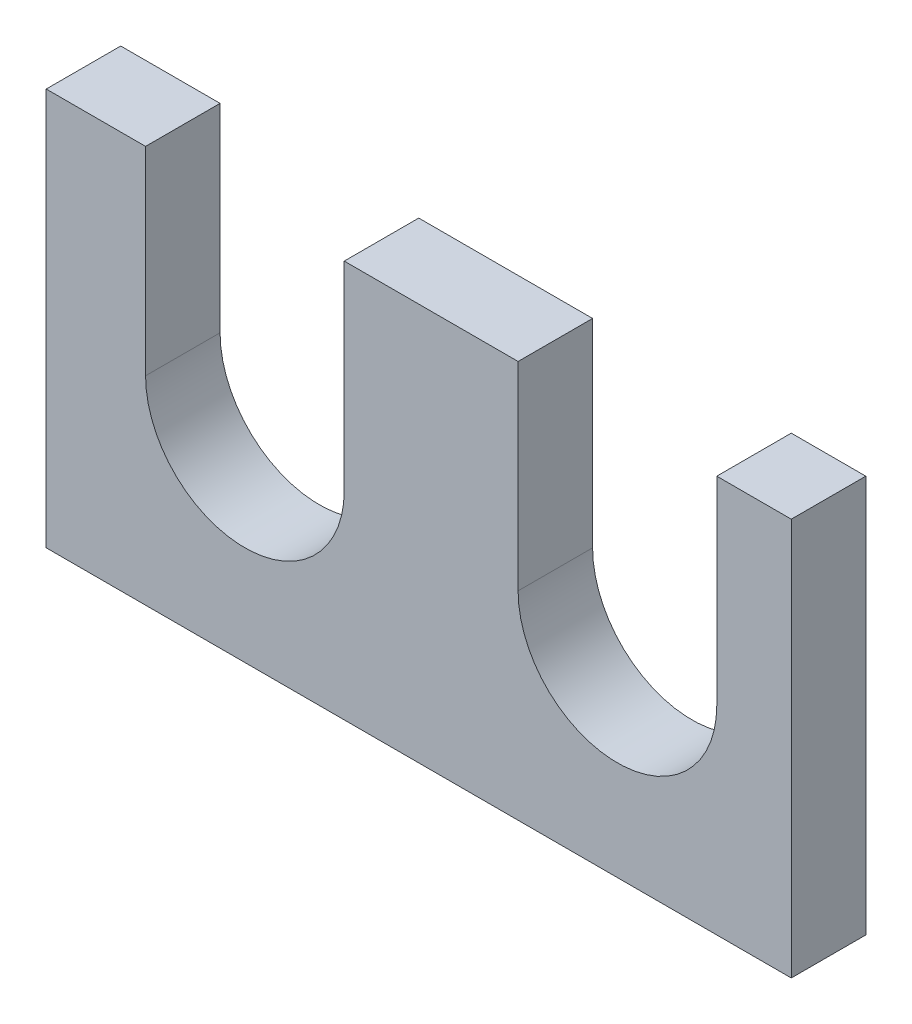
SolidWorks part; units mm, degrees
ref_plane "Front Plane" through (0, 0, 0) normal (0, 0, 1) x (1, 0, 0)
ref_plane "Top Plane" through (0, 0, 0) normal (0, 1, 0) x (1, 0, 0)
ref_plane "Right Plane" through (0, 0, 0) normal (1, 0, 0) x (0, 0, -1)
sketch "Sketch1" plane through (0, 0, 0) normal (0, 0, 1) x (1, 0, 0)
  line L0 (0, 8) -> (30, 8) construction
  line L1 (0, 0) -> (30, 0)
  line L2 (0, 0) -> (0, 16)
  line L3 (0, 16) -> (4, 16)
  line L4 (30, 0) -> (30, 16)
  line L5 (4, 8) -> (4, 16)
  line L6 (27, 16) -> (30, 16)
  line L7 (12, 8) -> (12, 16)
  line L9 (19, 8) -> (19, 16)
  line L11 (27, 8) -> (27, 16)
  line L12 (12, 16) -> (19, 16)
  arc A0 (4, 8) -> (12, 8) centre (8, 8) ccw
  arc A1 (19, 8) -> (27, 8) centre (23, 8) ccw
  dimension "D3" = 15
  dimension "D4" = 7
  dimension "D5" = 4
  dimension "D6" = 4
  dimension "D1" = 30
  dimension "D2" = 16
extrude "Boss-Extrude1" add sketch "Sketch1" along normal blind 3
